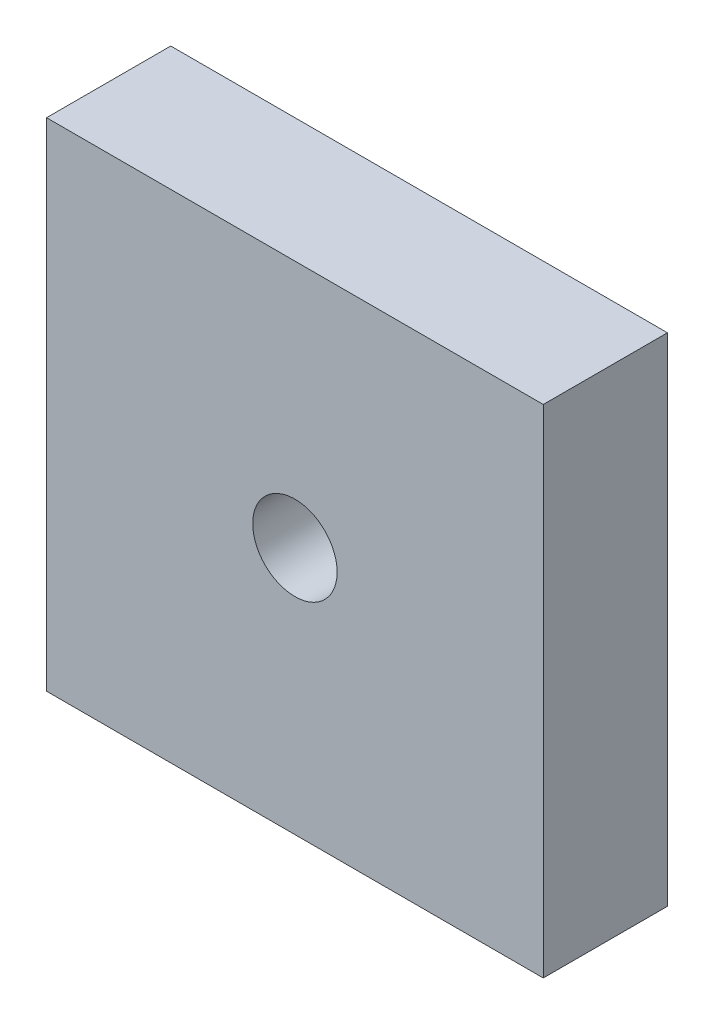
SolidWorks part; units mm, degrees
ref_plane "前视基准面" through (0, 0, 0) normal (0, 0, 1) x (1, 0, 0)
ref_plane "上视基准面" through (0, 0, 0) normal (0, 1, 0) x (1, 0, 0)
ref_plane "右视基准面" through (0, 0, 0) normal (1, 0, 0) x (0, 0, -1)
sketch "草图1" plane through (0, 0, 0) normal (0, 0, 1) x (1, 0, 0)
  line L1 (-20, -20) -> (20, -20)
  line L2 (-20, -20) -> (-20, 20)
  line L3 (-20, 20) -> (20, 20)
  line L4 (20, -20) -> (20, 20)
  line L5 (-20, -20) -> (20, 20) construction
  line L6 (-20, 20) -> (20, -20) construction
  point P0 (0, 0)
  dimension "D1" = 40
  dimension "D2" = 40
extrude "凸台-拉伸1" add sketch "草图1" along normal mid plane 10
hole_wizard "M8 螺纹孔1" positions "草图2" profile "草图3" tap size "M8" standard "GB" end condition through all
sketch "草图2" plane through (0, 0, 5) normal (0, 0, 1) x (1, 0, 0)
  line L0 (-20, 20) -> (-20, -20) construction
  line L1 (-20, -20) -> (20, -20) construction
  point P0 (0, 0)
  dimension "D1" = 20
  dimension "D2" = 20
sketch "草图3" plane through (0, 0, 5) normal (1, 0, 0) x (0, -1, 0)
  line L0 (0, 0) -> (0, 10)
  line L1 (0, 10) -> (3.4, 10)
  line L2 (3.4, 10) -> (3.4, 0)
  line L5 (3.4, 0) -> (0, 0)
  line L11 (0, -6.35) -> (0, 107.95) construction
  dimension "通孔螺纹孔钻头直径" = 6.8
  dimension "通孔螺纹孔钻头深度" = 10
cosmetic thread "孔螺蚊线1"
